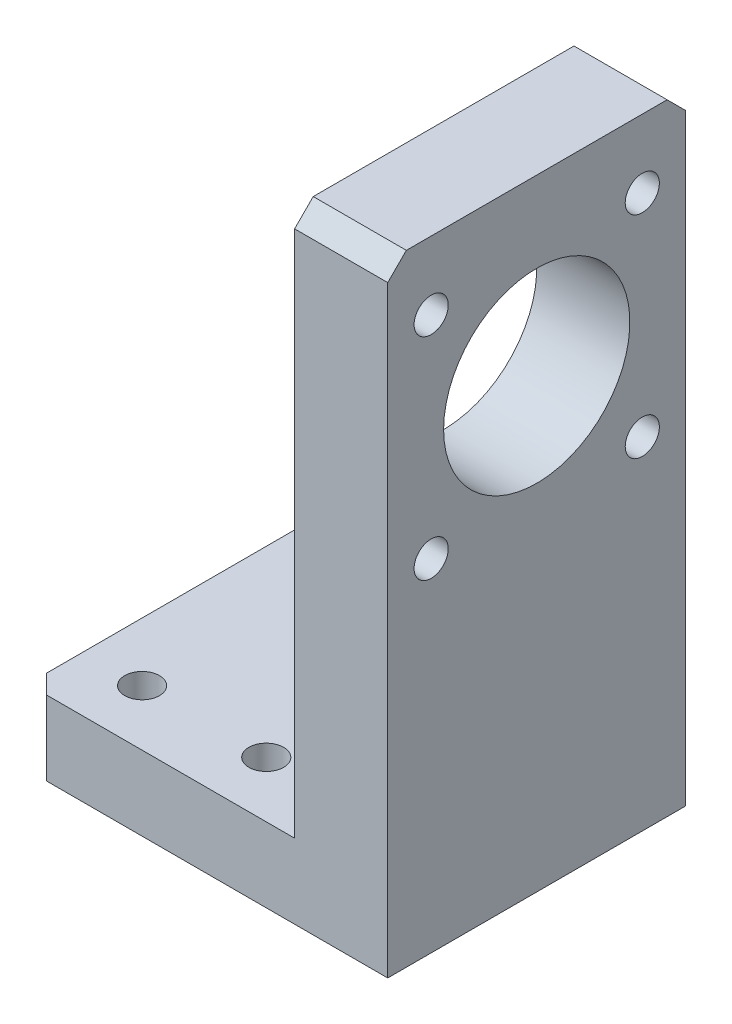
from build123d import *

# Parameters (mm, degrees)
BOSS_EXTRUDE1_DEPTH                                = 48
SKETCH2_R                                          = 15
CUT_EXTRUDE1_DEPTH                                 = 93.349417704
HOLE_SIZE_PER_HEX_SOCKET_CAP_SCREW_TYP_D           = 5.5
HOLE_SIZE_PER_HEX_SOCKET_CAP_SCREW_TYP_CBORE_D     = 10
HOLE_SIZE_PER_HEX_SOCKET_CAP_SCREW_TYP_CBORE_DEPTH = 5.7
CHAMFER1_SIZE                                      = 3
SKETCH6_R                                          = 2.8
CUT_EXTRUDE2_DEPTH                                 = 48


with BuildPart() as part:
    # Sketch1 → Boss-Extrude1 (new body)
    with BuildSketch(Plane.XY):
        Polygon((-9.247374932, 66.146919431), (-9.247374932, -21.853080569), (-52.247374932, -21.853080569), (-52.247374932, -33.853080569), (5.752625068, -33.853080569), (5.752625068, 66.146919431), align=None)
    extrude(amount=BOSS_EXTRUDE1_DEPTH)

    # Sketch2 → Cut-Extrude1 (cut, through all)
    with BuildSketch(Plane.ZY.offset(9.247374932)):
        with Locations((24, 38.146919431)):
            Circle(SKETCH2_R)
    extrude(amount=-CUT_EXTRUDE1_DEPTH, mode=Mode.SUBTRACT)

    # Hole size (per) hex socket cap screw type 1 (through all)
    with Locations(Plane.ZY.offset(9.247374932)):
        with Locations((7, 55.146919431), (41, 55.146919431), (41, 21.146919431), (7, 21.146919431)):
            CounterBoreHole(HOLE_SIZE_PER_HEX_SOCKET_CAP_SCREW_TYP_D / 2, HOLE_SIZE_PER_HEX_SOCKET_CAP_SCREW_TYP_CBORE_D / 2, HOLE_SIZE_PER_HEX_SOCKET_CAP_SCREW_TYP_CBORE_DEPTH)

    # Chamfer1
    chamfer1_edges = [part.edges().sort_by_distance(p)[0] for p in [
        (-52.247374932, -27.853080569, 48),
        (-1.747374932, 66.146919431, 48),
        (-52.247374932, -27.853080569, 0),
        (-1.747374932, 66.146919431, 0),
    ]]
    chamfer(chamfer1_edges, length=CHAMFER1_SIZE)

    # Sketch6 → Cut-Extrude2 (cut)
    with BuildSketch(Plane(origin=(0, -21.853080569, 0), x_dir=(1, 0, 0), z_dir=(0, 1, 0))):
        with Locations(Location((-42.810470963, -9, 0), (0, 0, 180))):
            Circle(SKETCH6_R)
        with Locations(Location((-22.810470963, -9, 0), (0, 0, 180))):
            Circle(SKETCH6_R)
        with Locations(Location((-42.810470963, -39, 0), (0, 0, 180))):
            Circle(SKETCH6_R)
        with Locations(Location((-22.810470963, -39, 0), (0, 0, 180))):
            Circle(SKETCH6_R)
    extrude(amount=-CUT_EXTRUDE2_DEPTH, mode=Mode.SUBTRACT)


solid = part.part
